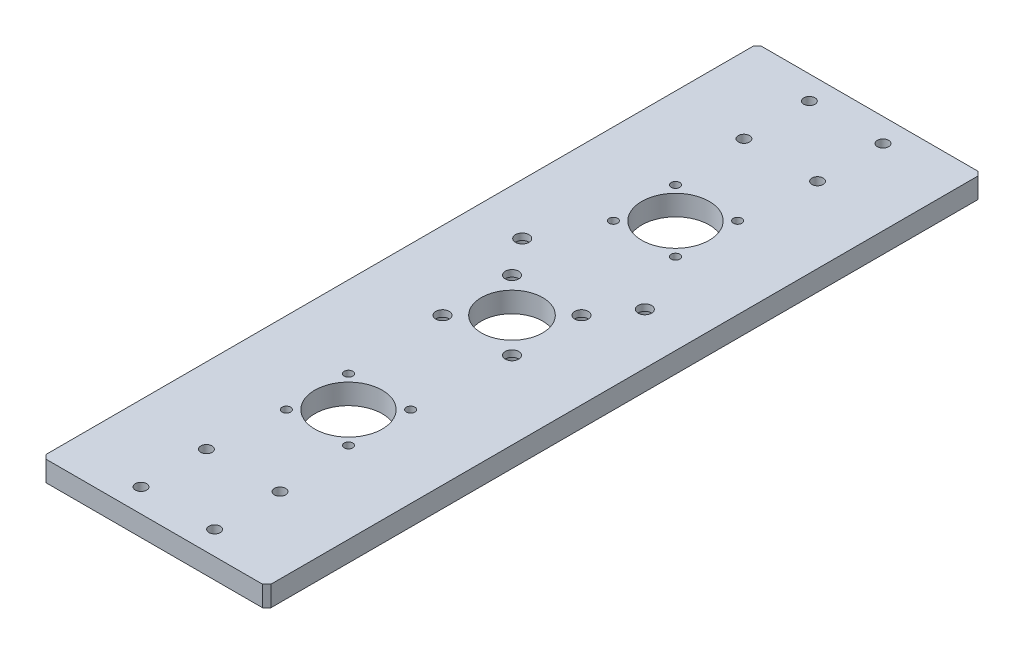
from build123d import *

# Parameters (mm, degrees)
SKETCH1_W                                         = 110
SKETCH1_H                                         = 350
BOSS_EXTRUDE1_DEPTH                               = 10
HOLE_SIZE_BY_SOCKET_HEAD_CAP_SCREW_TY_D           = 5.5
HOLE_SIZE_BY_SOCKET_HEAD_CAP_SCREW_TY_CBORE_D     = 10
HOLE_SIZE_BY_SOCKET_HEAD_CAP_SCREW_TY_CBORE_DEPTH = 5.7
HOLE_SIZE_BY_SOCKET_HEAD_CAP_SCRE_2_D             = 6.6
HOLE_SIZE_BY_SOCKET_HEAD_CAP_SCRE_2_CBORE_D       = 11
HOLE_SIZE_BY_SOCKET_HEAD_CAP_SCRE_2_CBORE_DEPTH   = 6.8
CHAMFER1_SIZE                                     = 2
HOLE_SIZE_BY_SOCKET_HEAD_CAP_SCRE_3_D             = 6.6
HOLE_SIZE_BY_SOCKET_HEAD_CAP_SCRE_3_CBORE_D       = 11
HOLE_SIZE_BY_SOCKET_HEAD_CAP_SCRE_3_CBORE_DEPTH   = 6.8
SKETCH8_R                                         = 16.5
CUT_EXTRUDE1_DEPTH                                = 184.711730709
M5_TAPPED_HOLE1_D                                 = 4.2
SKETCH11_R                                        = 15
CUT_EXTRUDE2_DEPTH                                = 184.711730709


with BuildPart() as part:
    # Sketch1 → Boss-Extrude1 (new body)
    with BuildSketch(Plane(origin=(0, 0, 0), x_dir=(1, 0, 0), z_dir=(0, 1, 0))):
        Rectangle(SKETCH1_W, SKETCH1_H)
    extrude(amount=BOSS_EXTRUDE1_DEPTH)

    # Hole Size _ by_ Socket Head Cap Screw Ty (through all)
    with Locations(Plane.XZ):
        with Locations((-18, 131.5), (18, 131.5), (18, 163.5), (-18, 163.5), (-18, -163.5), (-18, -131.5), (18, -163.5), (18, -131.5)):
            CounterBoreHole(HOLE_SIZE_BY_SOCKET_HEAD_CAP_SCREW_TY_D / 2, HOLE_SIZE_BY_SOCKET_HEAD_CAP_SCREW_TY_CBORE_D / 2, HOLE_SIZE_BY_SOCKET_HEAD_CAP_SCREW_TY_CBORE_DEPTH)

    # Hole Size _ by_ Socket Head Cap Scre 2 (through all)
    with Locations(Plane.XZ):
        with Locations((-17, -17), (17, -17), (17, 17), (-17, 17)):
            CounterBoreHole(HOLE_SIZE_BY_SOCKET_HEAD_CAP_SCRE_2_D / 2, HOLE_SIZE_BY_SOCKET_HEAD_CAP_SCRE_2_CBORE_D / 2, HOLE_SIZE_BY_SOCKET_HEAD_CAP_SCRE_2_CBORE_DEPTH)

    # Chamfer1
    chamfer1_edges = [part.edges().sort_by_distance(p)[0] for p in [
        (55, 5, 175),
        (-55, 5, 175),
        (-55, 5, -175),
        (55, 5, -175),
    ]]
    chamfer(chamfer1_edges, length=CHAMFER1_SIZE)

    # Hole Size _ by_ Socket Head Cap Scre 3 (through all)
    with Locations(Plane(origin=(0, 0, 0), x_dir=(-1, 0, 0), z_dir=(0, -1, 0))):
        with Locations((30, 35), (-30, 35)):
            CounterBoreHole(HOLE_SIZE_BY_SOCKET_HEAD_CAP_SCRE_3_D / 2, HOLE_SIZE_BY_SOCKET_HEAD_CAP_SCRE_3_CBORE_D / 2, HOLE_SIZE_BY_SOCKET_HEAD_CAP_SCRE_3_CBORE_DEPTH)

    # Sketch8 → Cut-Extrude1 (cut, through all)
    with BuildSketch(Plane.XZ):
        with Locations(Location((0, -80, 0), (0, 0, 270))):
            Circle(SKETCH8_R)
        with Locations(Location((0, 80, 0), (0, 0, 270))):
            Circle(SKETCH8_R)
    extrude(amount=-CUT_EXTRUDE1_DEPTH, mode=Mode.SUBTRACT)

    # M5 Tapped Hole1 (through all)
    with Locations(Plane(origin=(0, 10, 0), x_dir=(1, 0, 0), z_dir=(0, 1, 0))):
        with Locations((-15.202795796, 95.202795796), (15.202795796, 64.797204204), (-15.202795796, 64.797204204), (15.202795796, 95.202795796), (-15.202795796, -64.797204204), (15.202795796, -95.202795796), (15.202795796, -64.797204204), (-15.202795796, -95.202795796)):
            Hole(M5_TAPPED_HOLE1_D / 2)

    # Sketch11 → Cut-Extrude2 (cut, through all)
    with BuildSketch(Plane(origin=(0, 10, 0), x_dir=(1, 0, 0), z_dir=(0, 1, 0))):
        with Locations(Location((0, 0, 0), (0, 0, 270))):
            Circle(SKETCH11_R)
    extrude(amount=-CUT_EXTRUDE2_DEPTH, mode=Mode.SUBTRACT)


solid = part.part
